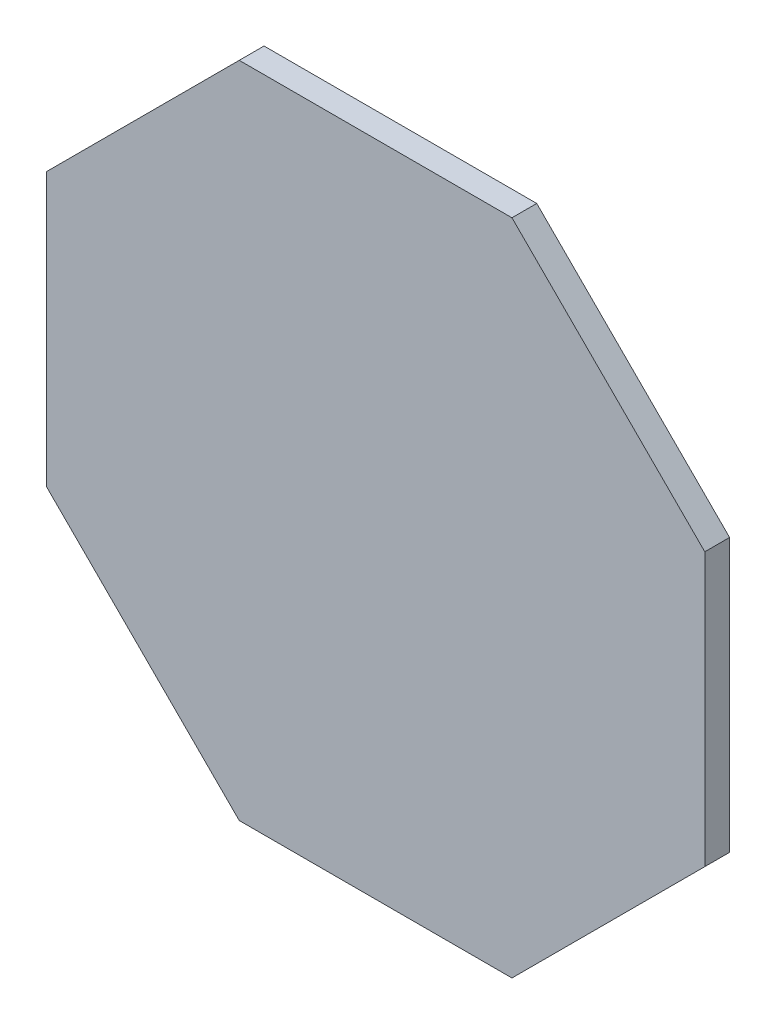
from build123d import *

# Parameters (mm, degrees)
SKETCH1_R             = 25
SKETCH1_R_2           = 20
BOSS_EXTRUDE1_DEPTH   = 10
BOSS_EXTRUDE1_2_DEPTH = 10
BOSS_EXTRUDE1_3_DEPTH = 10
BOSS_EXTRUDE2_DEPTH   = 10


with BuildPart() as part:
    # Sketch1 → Boss-Extrude1 (new body)
    with BuildSketch(Plane.XY):
        with Locations((-659.884196758, -20)):
            Circle(SKETCH1_R)
        with Locations((-659.884196758, -20)):
            Circle(SKETCH1_R_2, mode=Mode.SUBTRACT)
    extrude(amount=-BOSS_EXTRUDE1_DEPTH)



with BuildPart() as body_2:
    # Sketch1 → Boss-Extrude1 2 (new body)
    with BuildSketch(Plane.XY):
        with Locations((-539.884196758, -20)):
            Circle(SKETCH1_R)
        with Locations((-539.884196758, -20)):
            Circle(SKETCH1_R_2, mode=Mode.SUBTRACT)
    extrude(amount=-BOSS_EXTRUDE1_2_DEPTH)


with BuildPart() as body_3:
    # Sketch1 → Boss-Extrude1 3 (new body)
    with BuildSketch(Plane.XY):
        with Locations((-539.884196758, -160)):
            Circle(SKETCH1_R)
        with Locations((-539.884196758, -160)):
            Circle(SKETCH1_R_2, mode=Mode.SUBTRACT)
    extrude(amount=-BOSS_EXTRUDE1_3_DEPTH)


with BuildPart() as part_1:
    add(part.part)

    add(body_2.part)  # Boss-Extrude2 merges body 2

    add(body_3.part)  # Boss-Extrude2 merges body 3
    # Sketch2 → Boss-Extrude2 (add)
    with BuildSketch(Plane.XY):
        Polygon((-544.884196758, -222.781745931), (-467.102450828, -145), (-467.102450828, -35), (-544.884196758, 42.781745931), (-654.884196758, 42.781745931), (-732.665942689, -35), (-732.665942689, -145), (-654.884196758, -222.781745931), align=None)
    extrude(amount=BOSS_EXTRUDE2_DEPTH)


solid = part_1.part
